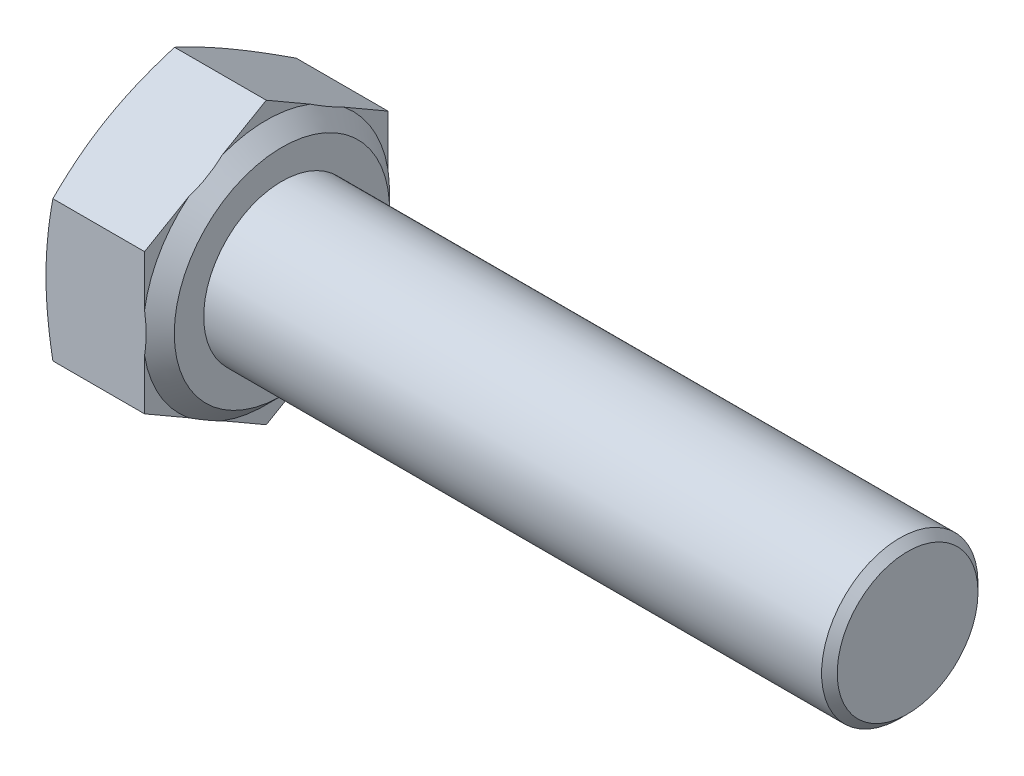
SolidWorks part; units mm, degrees
ref_plane "Front" through (0, 0, 0) normal (0, 0, 1) x (1, 0, 0)
ref_plane "Top" through (0, 0, 0) normal (0, 1, 0) x (1, 0, 0)
ref_plane "Right" through (0, 0, 0) normal (1, 0, 0) x (0, 0, -1)
sketch "Sketch2" plane through (0, 0, 0) normal (1, 0, 0) x (0, 0, -1)
  line L1 (3.89, -2.2459) -> (3.89, 2.2459)
  line L2 (3.89, 2.2459) -> (0, 4.4918)
  line L3 (0, 4.4918) -> (-3.89, 2.2459)
  line L4 (-3.89, 2.2459) -> (-3.89, -2.2459)
  line L5 (-3.89, -2.2459) -> (0, -4.4918)
  line L6 (0, -4.4918) -> (3.89, -2.2459)
  circle A0 centre (0, 0) radius 3.89 construction
extrude "BaseHead" add sketch "Sketch2" along normal blind 3.65
sketch "Sketch3" plane through (0, 0, 0) normal (0, 0, 1) x (1, 0, 0)
  line L0 (3.65, 4.4918) -> (3.65, 3.44)
  line L2 (3.65, 3.44) -> (3.15, 3.94)
  line L3 (3.15, 3.94) -> (3.15, 4.4918)
  line L5 (3.15, 4.4918) -> (3.65, 4.4918)
  line L6 (-0.9571, 0) -> (7.6478, 0) construction
  line L7 (3.65, 4.4918) -> (0, 4.4918) construction
  dimension "D1" = 45
  dimension "c" = 0.5
  dimension "Dw" = 6.88
revolve "BearingFace" cut sketch "Sketch3" angle 360 about L6
sketch "Sketch4" plane through (0, 0, 0) normal (0, 0, 1) x (1, 0, 0)
  line L0 (-0.4935, 0) -> (3.5626, 0) construction
  line L2 (0, 4.4918) -> (0.219, 4.4918)
  line L4 (0.219, 4.4918) -> (0, 3.89)
  line L6 (0, 3.89) -> (0, 4.4918)
  line L7 (3.15, 4.4918) -> (0, 4.4918) construction
revolve "HeadChamfer" cut sketch "Sketch4" angle 360 about L0
sketch "Sketch5" plane through (3.65, 0, 0) normal (1, 0, 0) x (0, 0, -1)
  circle A0 centre (0, 0) radius 2.5
extrude "BaseBody" add sketch "Sketch5" along normal blind 20
cosmetic thread "ThreadCosmetic1" [suppressed] parameters "D2"=4.134
chamfer "Chamfer1" distance 0.25 angle 45 1 edges at (23.65, 0, -2.5)
fillet "HeadFillet" [suppressed] radius 0.2
sketch "Sketch6" plane through (0, 0, 0) normal (0, 0, 1) x (1, 0, 0)
  line L0 (3.65, 2.933) -> (4.083, 2.933)
  line L1 (4.083, 2.933) -> (4.083, 2.5)
  line L2 (4.083, 2.5) -> (3.8665, 2.125)
  line L3 (3.8665, 2.125) -> (3.65, 2.5)
  line L4 (3.65, 2.5) -> (3.65, 2.933)
  line L5 (23.4, 2.5) -> (3.65, 2.5) construction
  line L6 (3.65, -3.44) -> (3.65, 3.44) construction
revolve "Cut-Revolve10" [suppressed] cut sketch "Sketch6" angle 360 about axis through (-0.9571, 0, 0) along (1, 0, 0)
pattern_linear "LPattern10" [suppressed] count 38
equation "\"D2@Sketch4\" = \"s@Sketch2\""
equation "\"D1@Chamfer1\" = 0.05 * \"d@Sketch5\""
equation "\"D1@Sketch6\" =  ( \"d@Sketch5\" - \"D2@ThreadCosmetic1\" )  / 2"
equation "\"pitch@LPattern10\" = \"D1@Sketch6\" * 1.2"
equation "\"D1@LPattern10\" = \"l@BaseBody\" / \"pitch@LPattern10\""
